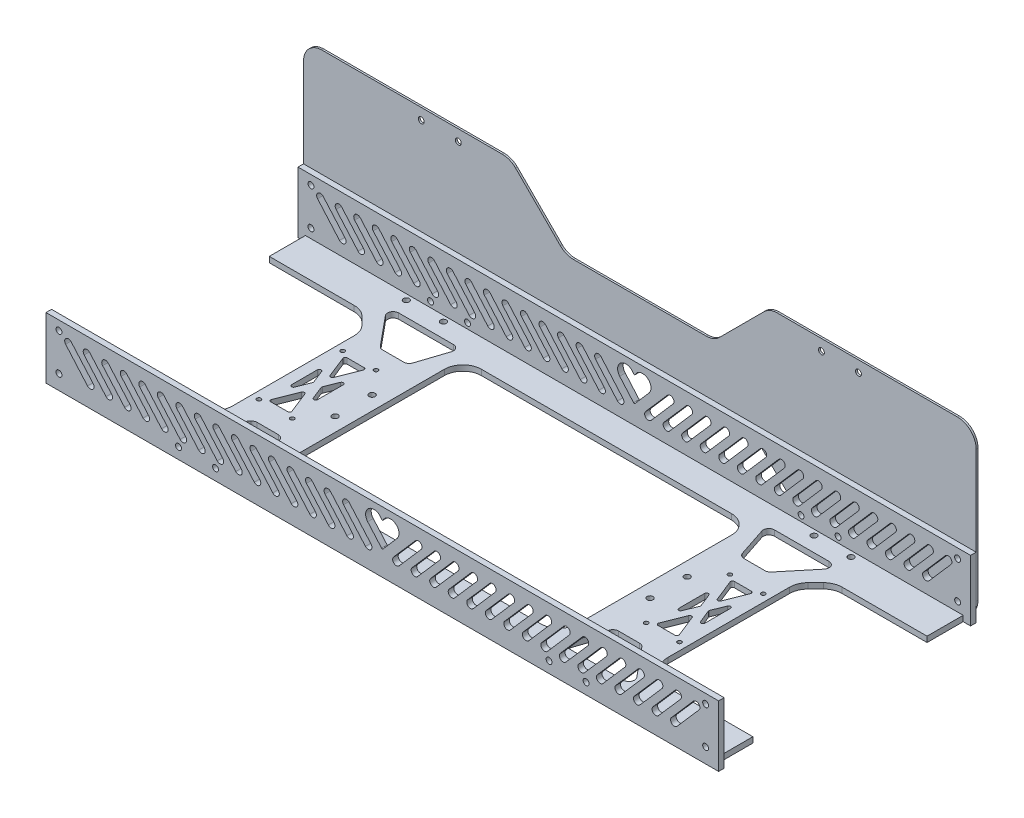
SolidWorks part; units mm, degrees
material "哈碳纤"
ref_plane "前视基准面" through (0, 0, 0) normal (0, 0, 1) x (1, 0, 0)
ref_plane "上视基准面" through (0, 0, 0) normal (0, 1, 0) x (1, 0, 0)
ref_plane "右视基准面" through (0, 0, 0) normal (1, 0, 0) x (0, 0, -1)
other "Configuration Table"
sketch "草图1" plane through (0, 0, 0) normal (0, 1, 0) x (1, 0, 0)
  line L0 (0, 66.5) -> (0, -66.5) construction
  line L1 (-177.5, -66.5) -> (177.5, -66.5)
  line L2 (-177.5, -66.5) -> (-177.5, 66.5)
  line L3 (-177.5, 66.5) -> (177.5, 66.5)
  line L4 (177.5, -66.5) -> (177.5, 66.5)
  line L5 (-177.5, -66.5) -> (177.5, 66.5) construction
  line L6 (-177.5, 66.5) -> (177.5, -66.5) construction
  line L7 (-1000, 0) -> (49000, 0) construction
  circle A4 centre (-120, -63.5) radius 1.6
  circle A5 centre (120, -63.5) radius 1.6
  circle A6 centre (-100, -63.5) radius 1.6
  circle A7 centre (100, -63.5) radius 1.6
  circle A8 centre (100, 63.5) radius 1.6
  circle A9 centre (-100, 63.5) radius 1.6
  circle A10 centre (120, 63.5) radius 1.6
  circle A11 centre (-120, 63.5) radius 1.6
  point P0 (0, 0)
  dimension "D3" = 3
  dimension "D4" = 3.2
  dimension "D1" = 133
  dimension "D2" = 355
  dimension "D5" = 20
  dimension "D6" = 200
extrude "凸台-拉伸1" add sketch "草图1" along normal blind 3
sketch "草图2" plane through (0, 0, 66.5) normal (0, 0, 1) x (1, 0, 0)
  line L1 (-181.5, 0) -> (181.5, 0)
  line L2 (-181.5, 0) -> (-181.5, 33)
  line L3 (-181.5, 33) -> (181.5, 33)
  line L4 (181.5, 0) -> (181.5, 33)
  line L5 (0, 0) -> (0, 33) construction
  line L7 (-100, 3) -> (-100, 0) construction
  line L8 (-177.5, 0) -> (177.5, 0) construction
  circle A0 centre (-174.5, 28) radius 1.6
  circle A1 centre (174.5, 28) radius 1.6
  circle A2 centre (-174.5, 8) radius 1.6
  circle A3 centre (174.5, 8) radius 1.6
  circle A4 centre (-110, 6) radius 1.6
  circle A5 centre (110, 6) radius 1.6
  circle A6 centre (-90, 6) radius 1.6
  circle A7 centre (90, 6) radius 1.6
  dimension "D2" = 7
  dimension "D3" = 3.2
  dimension "D6" = 6
  dimension "D7" = 3.2
  dimension "D1" = 33
  dimension "D4" = 20
  dimension "D5" = 8
  dimension "D8" = 20
  dimension "D9" = 10
  dimension "D10" = 363
extrude "凸台-拉伸2" add sketch "草图2" along normal blind 3 separate body
mirror "镜向1" about plane through (0, 0, 0) normal (0, 0, 1) of bodies 107
sketch "草图3" plane through (0, 3, 0) normal (0, 1, 0) x (1, 0, 0)
  line L0 (0, -1000) -> (0, 49000) construction
  line L1 (-177.5, 47) -> (-127.5, 47)
  line L2 (-177.5, 66.5) -> (-177.5, -66.5) construction
  line L3 (177.5, 47) -> (127.5, 47)
  line L4 (-127.5, 47) -> (-117.5, 37)
  line L5 (127.5, 47) -> (117.5, 37)
  line L6 (-117.5, 37) -> (-117.5, -37)
  line L7 (117.5, 37) -> (117.5, -37)
  line L8 (-117.5, -37) -> (-127.5, -47)
  line L9 (117.5, -37) -> (127.5, -47)
  line L10 (-127.5, -47) -> (-177.5, -47)
  line L11 (127.5, -47) -> (177.5, -47)
  line L12 (-177.5, -47) -> (-177.5, 47)
  line L13 (177.5, -47) -> (177.5, 47)
  line L14 (-177.5, -66.5) -> (177.5, -66.5) construction
  line L15 (-67.5, -51.5) -> (67.5, -51.5)
  line L16 (-77.5, -41.5) -> (-77.5, 41.5)
  line L17 (-67.5, 51.5) -> (67.5, 51.5)
  line L18 (77.5, -41.5) -> (77.5, 41.5)
  line L19 (-77.5, -51.5) -> (77.5, 51.5) construction
  line L20 (-77.5, 51.5) -> (77.5, -51.5) construction
  line L21 (181.5, -66.5) -> (-181.5, -66.5) construction
  line L22 (-85, 10) -> (-85, -10) construction
  line L23 (85, 10) -> (85, -10) construction
  line L24 (95.5, -22.6) -> (95.5, 22.6) construction
  line L25 (-113.5, -22.6) -> (-95.5, -22.6) construction
  line L26 (-113.5, -22.6) -> (-113.5, 22.6) construction
  line L27 (-113.5, 22.6) -> (-95.5, 22.6) construction
  line L28 (-95.5, -22.6) -> (-95.5, 22.6) construction
  line L29 (113.5, 22.6) -> (95.5, 22.6) construction
  line L30 (113.5, -22.6) -> (113.5, 22.6) construction
  line L31 (113.5, -22.6) -> (95.5, -22.6) construction
  arc A0 (-67.5, -51.5) -> (-77.5, -41.5) centre (-67.5, -41.5) cw
  arc A1 (-77.5, 41.5) -> (-67.5, 51.5) centre (-67.5, 41.5) cw
  arc A2 (67.5, 51.5) -> (77.5, 41.5) centre (67.5, 41.5) cw
  arc A3 (67.5, -51.5) -> (77.5, -41.5) centre (67.5, -41.5) ccw
  circle A4 centre (-85, 10) radius 1.6
  circle A5 centre (-85, -10) radius 1.6
  circle A6 centre (85, -10) radius 1.6
  circle A7 centre (85, 10) radius 1.6
  circle A8 centre (-113.5, 22.6) radius 1.1
  circle A9 centre (-95.5, 22.6) radius 1.1
  circle A11 centre (-113.5, -22.6) radius 1.1
  circle A12 centre (-95.5, -22.6) radius 1.1
  circle A13 centre (95.5, -22.6) radius 1.1
  circle A14 centre (113.5, -22.6) radius 1.1
  circle A15 centre (95.5, 22.6) radius 1.1
  circle A16 centre (113.5, 22.6) radius 1.1
  point P17 (-177.5, 0)
  point P18 (0, 0)
  point P43 (-85, 0)
  point P52 (-95.5, 0)
  dimension "D6" = 10
  dimension "D7" = 3.2
  dimension "D13" = 2.2
  dimension "D1" = 19.5
  dimension "D2" = 60
  dimension "D3" = 50
  dimension "D4" = 40
  dimension "D5" = 15
  dimension "D8" = 20
  dimension "D9" = 170
  dimension "D10" = 45.2
  dimension "D11" = 18
  dimension "D12" = 4
extrude "切除-拉伸1" cut sketch "草图3" against normal blind 10
fillet "圆角1" radius 10 8 edges at (127.5, 1.5, 47) (117.5, 1.5, 37) (117.5, 1.5, -37) (-127.5, 1.5, 47) (-117.5, 1.5, 37) (-117.5, 1.5, -37) (-127.5, 1.5, -47) (127.5, 1.5, -47)
sketch "草图4" plane through (0, 0, 69.5) normal (0, 0, 1) x (1, 0, 0)
  line L0 (-169.4178, 24.7808) -> (-157.5822, 11.2192) construction
  line L1 (-167.911, 26.0959) -> (-156.0753, 12.5342)
  line L2 (-170.9247, 23.4658) -> (-159.089, 9.9041)
  line L3 (181.5, 33) -> (-181.5, 33) construction
  line L4 (-181.5, 33) -> (-181.5, 0) construction
  line L5 (-181.5, 0) -> (181.5, 0) construction
  line L6 (-159.4178, 24.7808) -> (-147.5822, 11.2192) construction
  line L7 (-157.911, 26.0959) -> (-146.0753, 12.5342)
  line L8 (-160.9247, 23.4658) -> (-149.089, 9.9041)
  line L9 (-149.4178, 24.7808) -> (-137.5822, 11.2192) construction
  line L10 (-147.911, 26.0959) -> (-136.0753, 12.5342)
  line L11 (-150.9247, 23.4658) -> (-139.089, 9.9041)
  line L12 (-139.4178, 24.7808) -> (-127.5822, 11.2192) construction
  line L13 (-137.911, 26.0959) -> (-126.0753, 12.5342)
  line L14 (-140.9247, 23.4658) -> (-129.089, 9.9041)
  line L15 (-129.4178, 24.7808) -> (-117.5822, 11.2192) construction
  line L16 (-127.911, 26.0959) -> (-116.0753, 12.5342)
  line L17 (-130.9247, 23.4658) -> (-119.089, 9.9041)
  line L18 (-119.4178, 24.7808) -> (-107.5822, 11.2192) construction
  line L19 (-117.911, 26.0959) -> (-106.0753, 12.5342)
  line L20 (-120.9247, 23.4658) -> (-109.089, 9.9041)
  line L21 (-109.4178, 24.7808) -> (-97.5822, 11.2192) construction
  line L22 (-107.911, 26.0959) -> (-96.0753, 12.5342)
  line L23 (-110.9247, 23.4658) -> (-99.089, 9.9041)
  line L24 (-99.4178, 24.7808) -> (-87.5822, 11.2192) construction
  line L25 (-97.911, 26.0959) -> (-86.0753, 12.5342)
  line L26 (-100.9247, 23.4658) -> (-89.089, 9.9041)
  line L27 (-89.4178, 24.7808) -> (-77.5822, 11.2192) construction
  line L28 (-87.911, 26.0959) -> (-76.0753, 12.5342)
  line L29 (-90.9247, 23.4658) -> (-79.089, 9.9041)
  line L30 (-79.4178, 24.7808) -> (-67.5822, 11.2192) construction
  line L31 (-77.911, 26.0959) -> (-66.0753, 12.5342)
  line L32 (-80.9247, 23.4658) -> (-69.089, 9.9041)
  line L33 (-69.4178, 24.7808) -> (-57.5822, 11.2192) construction
  line L34 (-67.911, 26.0959) -> (-56.0753, 12.5342)
  line L35 (-70.9247, 23.4658) -> (-59.089, 9.9041)
  line L36 (-59.4178, 24.7808) -> (-47.5822, 11.2192) construction
  line L37 (-57.911, 26.0959) -> (-46.0753, 12.5342)
  line L38 (-60.9247, 23.4658) -> (-49.089, 9.9041)
  line L39 (-49.4178, 24.7808) -> (-37.5822, 11.2192) construction
  line L40 (-47.911, 26.0959) -> (-36.0753, 12.5342)
  line L41 (-50.9247, 23.4658) -> (-39.089, 9.9041)
  line L42 (-39.4178, 24.7808) -> (-27.5822, 11.2192) construction
  line L43 (-37.911, 26.0959) -> (-26.0753, 12.5342)
  line L44 (-40.9247, 23.4658) -> (-29.089, 9.9041)
  line L45 (-29.4178, 24.7808) -> (-17.5822, 11.2192) construction
  line L46 (-27.911, 26.0959) -> (-16.0753, 12.5342)
  line L47 (-30.9247, 23.4658) -> (-19.089, 9.9041)
  line L48 (-19.4178, 24.7808) -> (-7.5822, 11.2192) construction
  line L49 (-17.911, 26.0959) -> (-6.0753, 12.5342)
  line L50 (-20.9247, 23.4658) -> (-9.089, 9.9041)
  line L51 (-169.4178, 24.7808) -> (-159.4178, 24.7808) construction
  line L52 (0, 33) -> (0, 0) construction
  line L53 (169.4178, 24.7808) -> (157.5822, 11.2192) construction
  line L54 (167.911, 26.0959) -> (156.0753, 12.5342)
  line L55 (170.9247, 23.4658) -> (159.089, 9.9041)
  line L56 (159.4178, 24.7808) -> (147.5822, 11.2192) construction
  line L57 (157.911, 26.0959) -> (146.0753, 12.5342)
  line L58 (160.9247, 23.4658) -> (149.089, 9.9041)
  line L59 (149.4178, 24.7808) -> (137.5822, 11.2192) construction
  line L60 (147.911, 26.0959) -> (136.0753, 12.5342)
  line L61 (150.9247, 23.4658) -> (139.089, 9.9041)
  line L62 (139.4178, 24.7808) -> (127.5822, 11.2192) construction
  line L63 (137.911, 26.0959) -> (126.0753, 12.5342)
  line L64 (140.9247, 23.4658) -> (129.089, 9.9041)
  line L65 (129.4178, 24.7808) -> (117.5822, 11.2192) construction
  line L66 (127.911, 26.0959) -> (116.0753, 12.5342)
  line L67 (130.9247, 23.4658) -> (119.089, 9.9041)
  line L68 (119.4178, 24.7808) -> (107.5822, 11.2192) construction
  line L69 (117.911, 26.0959) -> (106.0753, 12.5342)
  line L70 (120.9247, 23.4658) -> (109.089, 9.9041)
  line L71 (109.4178, 24.7808) -> (97.5822, 11.2192) construction
  line L72 (107.911, 26.0959) -> (96.0753, 12.5342)
  line L73 (110.9247, 23.4658) -> (99.089, 9.9041)
  line L74 (99.4178, 24.7808) -> (87.5822, 11.2192) construction
  line L75 (97.911, 26.0959) -> (86.0753, 12.5342)
  line L76 (100.9247, 23.4658) -> (89.089, 9.9041)
  line L77 (89.4178, 24.7808) -> (77.5822, 11.2192) construction
  line L78 (87.911, 26.0959) -> (76.0753, 12.5342)
  line L79 (90.9247, 23.4658) -> (79.089, 9.9041)
  line L80 (79.4178, 24.7808) -> (67.5822, 11.2192) construction
  line L81 (77.911, 26.0959) -> (66.0753, 12.5342)
  line L82 (80.9247, 23.4658) -> (69.089, 9.9041)
  line L83 (69.4178, 24.7808) -> (57.5822, 11.2192) construction
  line L84 (67.911, 26.0959) -> (56.0753, 12.5342)
  line L85 (70.9247, 23.4658) -> (59.089, 9.9041)
  line L86 (59.4178, 24.7808) -> (47.5822, 11.2192) construction
  line L87 (57.911, 26.0959) -> (46.0753, 12.5342)
  line L88 (60.9247, 23.4658) -> (49.089, 9.9041)
  line L89 (49.4178, 24.7808) -> (37.5822, 11.2192) construction
  line L90 (47.911, 26.0959) -> (36.0753, 12.5342)
  line L91 (50.9247, 23.4658) -> (39.089, 9.9041)
  line L92 (39.4178, 24.7808) -> (27.5822, 11.2192) construction
  line L93 (37.911, 26.0959) -> (26.0753, 12.5342)
  line L94 (40.9247, 23.4658) -> (29.089, 9.9041)
  line L95 (29.4178, 24.7808) -> (17.5822, 11.2192) construction
  line L96 (27.911, 26.0959) -> (16.0753, 12.5342)
  line L97 (30.9247, 23.4658) -> (19.089, 9.9041)
  line L98 (19.4178, 24.7808) -> (7.5822, 11.2192) construction
  line L99 (17.911, 26.0959) -> (6.0753, 12.5342)
  line L100 (20.9247, 23.4658) -> (9.089, 9.9041)
  line L101 (169.4178, 24.7808) -> (159.4178, 24.7808) construction
  line L102 (-0.3767, 13.4316) -> (-7.8904, 22.0411)
  line L103 (0.3767, 13.4316) -> (7.8904, 22.0411)
  arc A0 (-167.911, 26.0959) -> (-170.9247, 23.4658) centre (-169.4178, 24.7808) ccw
  arc A1 (-159.089, 9.9041) -> (-156.0753, 12.5342) centre (-157.5822, 11.2192) ccw
  arc A2 (-157.911, 26.0959) -> (-160.9247, 23.4658) centre (-159.4178, 24.7808) ccw
  arc A3 (-149.089, 9.9041) -> (-146.0753, 12.5342) centre (-147.5822, 11.2192) ccw
  arc A4 (-147.911, 26.0959) -> (-150.9247, 23.4658) centre (-149.4178, 24.7808) ccw
  arc A5 (-139.089, 9.9041) -> (-136.0753, 12.5342) centre (-137.5822, 11.2192) ccw
  arc A6 (-137.911, 26.0959) -> (-140.9247, 23.4658) centre (-139.4178, 24.7808) ccw
  arc A7 (-129.089, 9.9041) -> (-126.0753, 12.5342) centre (-127.5822, 11.2192) ccw
  arc A8 (-127.911, 26.0959) -> (-130.9247, 23.4658) centre (-129.4178, 24.7808) ccw
  arc A9 (-119.089, 9.9041) -> (-116.0753, 12.5342) centre (-117.5822, 11.2192) ccw
  arc A10 (-117.911, 26.0959) -> (-120.9247, 23.4658) centre (-119.4178, 24.7808) ccw
  arc A11 (-109.089, 9.9041) -> (-106.0753, 12.5342) centre (-107.5822, 11.2192) ccw
  arc A12 (-107.911, 26.0959) -> (-110.9247, 23.4658) centre (-109.4178, 24.7808) ccw
  arc A13 (-99.089, 9.9041) -> (-96.0753, 12.5342) centre (-97.5822, 11.2192) ccw
  arc A14 (-97.911, 26.0959) -> (-100.9247, 23.4658) centre (-99.4178, 24.7808) ccw
  arc A15 (-89.089, 9.9041) -> (-86.0753, 12.5342) centre (-87.5822, 11.2192) ccw
  arc A16 (-87.911, 26.0959) -> (-90.9247, 23.4658) centre (-89.4178, 24.7808) ccw
  arc A17 (-79.089, 9.9041) -> (-76.0753, 12.5342) centre (-77.5822, 11.2192) ccw
  arc A18 (-77.911, 26.0959) -> (-80.9247, 23.4658) centre (-79.4178, 24.7808) ccw
  arc A19 (-69.089, 9.9041) -> (-66.0753, 12.5342) centre (-67.5822, 11.2192) ccw
  arc A20 (-67.911, 26.0959) -> (-70.9247, 23.4658) centre (-69.4178, 24.7808) ccw
  arc A21 (-59.089, 9.9041) -> (-56.0753, 12.5342) centre (-57.5822, 11.2192) ccw
  arc A22 (-57.911, 26.0959) -> (-60.9247, 23.4658) centre (-59.4178, 24.7808) ccw
  arc A23 (-49.089, 9.9041) -> (-46.0753, 12.5342) centre (-47.5822, 11.2192) ccw
  arc A24 (-47.911, 26.0959) -> (-50.9247, 23.4658) centre (-49.4178, 24.7808) ccw
  arc A25 (-39.089, 9.9041) -> (-36.0753, 12.5342) centre (-37.5822, 11.2192) ccw
  arc A26 (-37.911, 26.0959) -> (-40.9247, 23.4658) centre (-39.4178, 24.7808) ccw
  arc A27 (-29.089, 9.9041) -> (-26.0753, 12.5342) centre (-27.5822, 11.2192) ccw
  arc A28 (-27.911, 26.0959) -> (-30.9247, 23.4658) centre (-29.4178, 24.7808) ccw
  arc A29 (-19.089, 9.9041) -> (-16.0753, 12.5342) centre (-17.5822, 11.2192) ccw
  arc A30 (-17.911, 26.0959) -> (-20.9247, 23.4658) centre (-19.4178, 24.7808) ccw
  arc A31 (-9.089, 9.9041) -> (-6.0753, 12.5342) centre (-7.5822, 11.2192) ccw
  arc A32 (167.911, 26.0959) -> (170.9247, 23.4658) centre (169.4178, 24.7808) cw
  arc A33 (159.089, 9.9041) -> (156.0753, 12.5342) centre (157.5822, 11.2192) cw
  arc A34 (157.911, 26.0959) -> (160.9247, 23.4658) centre (159.4178, 24.7808) cw
  arc A35 (149.089, 9.9041) -> (146.0753, 12.5342) centre (147.5822, 11.2192) cw
  arc A36 (147.911, 26.0959) -> (150.9247, 23.4658) centre (149.4178, 24.7808) cw
  arc A37 (139.089, 9.9041) -> (136.0753, 12.5342) centre (137.5822, 11.2192) cw
  arc A38 (137.911, 26.0959) -> (140.9247, 23.4658) centre (139.4178, 24.7808) cw
  arc A39 (129.089, 9.9041) -> (126.0753, 12.5342) centre (127.5822, 11.2192) cw
  arc A40 (127.911, 26.0959) -> (130.9247, 23.4658) centre (129.4178, 24.7808) cw
  arc A41 (119.089, 9.9041) -> (116.0753, 12.5342) centre (117.5822, 11.2192) cw
  arc A42 (117.911, 26.0959) -> (120.9247, 23.4658) centre (119.4178, 24.7808) cw
  arc A43 (109.089, 9.9041) -> (106.0753, 12.5342) centre (107.5822, 11.2192) cw
  arc A44 (107.911, 26.0959) -> (110.9247, 23.4658) centre (109.4178, 24.7808) cw
  arc A45 (99.089, 9.9041) -> (96.0753, 12.5342) centre (97.5822, 11.2192) cw
  arc A46 (97.911, 26.0959) -> (100.9247, 23.4658) centre (99.4178, 24.7808) cw
  arc A47 (89.089, 9.9041) -> (86.0753, 12.5342) centre (87.5822, 11.2192) cw
  arc A48 (87.911, 26.0959) -> (90.9247, 23.4658) centre (89.4178, 24.7808) cw
  arc A49 (79.089, 9.9041) -> (76.0753, 12.5342) centre (77.5822, 11.2192) cw
  arc A50 (77.911, 26.0959) -> (80.9247, 23.4658) centre (79.4178, 24.7808) cw
  arc A51 (69.089, 9.9041) -> (66.0753, 12.5342) centre (67.5822, 11.2192) cw
  arc A52 (67.911, 26.0959) -> (70.9247, 23.4658) centre (69.4178, 24.7808) cw
  arc A53 (59.089, 9.9041) -> (56.0753, 12.5342) centre (57.5822, 11.2192) cw
  arc A54 (57.911, 26.0959) -> (60.9247, 23.4658) centre (59.4178, 24.7808) cw
  arc A55 (49.089, 9.9041) -> (46.0753, 12.5342) centre (47.5822, 11.2192) cw
  arc A56 (47.911, 26.0959) -> (50.9247, 23.4658) centre (49.4178, 24.7808) cw
  arc A57 (39.089, 9.9041) -> (36.0753, 12.5342) centre (37.5822, 11.2192) cw
  arc A58 (37.911, 26.0959) -> (40.9247, 23.4658) centre (39.4178, 24.7808) cw
  arc A59 (29.089, 9.9041) -> (26.0753, 12.5342) centre (27.5822, 11.2192) cw
  arc A60 (27.911, 26.0959) -> (30.9247, 23.4658) centre (29.4178, 24.7808) cw
  arc A61 (19.089, 9.9041) -> (16.0753, 12.5342) centre (17.5822, 11.2192) cw
  arc A62 (17.911, 26.0959) -> (20.9247, 23.4658) centre (19.4178, 24.7808) cw
  arc A63 (9.089, 9.9041) -> (6.0753, 12.5342) centre (7.5822, 11.2192) cw
  arc A64 (-0.45, 26.9615) -> (-7.8904, 22.0411) centre (-4.5, 25) ccw
  arc A65 (0.45, 26.9615) -> (7.8904, 22.0411) centre (4.5, 25) cw
  arc A66 (-0.3767, 13.4316) -> (0.3767, 13.4316) centre (0, 13.7604) ccw
  arc A67 (0.45, 26.9615) -> (-0.45, 26.9615) centre (0, 27.1794) cw
  point P2 (-163.5, 18)
  point P16 (-153.5, 18)
  point P23 (-143.5, 18)
  point P30 (-133.5, 18)
  point P37 (-123.5, 18)
  point P44 (-113.5, 18)
  point P51 (-103.5, 18)
  point P58 (-93.5, 18)
  point P65 (-83.5, 18)
  point P72 (-73.5, 18)
  point P79 (-63.5, 18)
  point P86 (-53.5, 18)
  point P93 (-43.5, 18)
  point P100 (-33.5, 18)
  point P107 (-23.5, 18)
  point P114 (-13.5, 18)
  point P125 (163.5, 18)
  point P132 (153.5, 18)
  point P139 (143.5, 18)
  point P146 (133.5, 18)
  point P153 (123.5, 18)
  point P160 (113.5, 18)
  point P167 (103.5, 18)
  point P174 (93.5, 18)
  point P181 (83.5, 18)
  point P188 (73.5, 18)
  point P195 (63.5, 18)
  point P202 (53.5, 18)
  point P209 (43.5, 18)
  point P216 (33.5, 18)
  point P223 (23.5, 18)
  point P230 (13.5, 18)
  point P243 (0, 13)
  point P248 (0, 25)
extrude "切除-拉伸2" cut sketch "草图4" against normal through all
sketch "草图6" plane through (0, 3, 0) normal (0, 1, 0) x (1, 0, 0)
  line L0 (-109.0762, -20.6) -> (-99.9238, -20.6)
  line L1 (-113.5, -22.6) -> (-95.5, -22.6) construction
  line L2 (-113.5, -22.6) -> (-113.5, 22.6) construction
  line L3 (-113.5, 22.6) -> (-95.5, 22.6) construction
  line L4 (-95.5, -22.6) -> (-95.5, 22.6) construction
  line L5 (-113.5, -22.6) -> (-95.5, 22.6) construction
  line L6 (-113.5, 22.6) -> (-95.5, -22.6) construction
  line L7 (-111.5, -6.958) -> (-111.5, 6.958)
  line L9 (-110.0052, -19.23) -> (-105.429, -7.7387)
  line L10 (-103.571, 7.7387) -> (-98.9948, 19.23)
  line L11 (-109.571, 7.3279) -> (-106.8001, 0.37)
  line L12 (-102.1999, 0.37) -> (-99.429, 7.3279)
  line L13 (-111.6419, 23.3399) -> (-93.6419, -21.8601) construction
  line L14 (-115.3581, -21.8601) -> (-97.3581, 23.3399) construction
  line L15 (-102.1999, -0.37) -> (-99.429, -7.3279)
  line L16 (-109.571, -7.3279) -> (-106.8001, -0.37)
  line L17 (-110.0052, 19.23) -> (-105.429, 7.7387)
  line L18 (-111.5, -22.6) -> (-111.5, 22.6) construction
  line L19 (-115.3581, 21.8601) -> (-97.3581, -23.3399) construction
  line L20 (-109.0762, 20.6) -> (-99.9238, 20.6)
  line L22 (-97.5, -6.958) -> (-97.5, 6.958)
  line L23 (-103.571, -7.7387) -> (-98.9948, -19.23)
  line L24 (-117.5, 32.8579) -> (-77.5, 32.8579) construction
  line L25 (-118.4432, 50.5893) -> (-105.5208, 34.9472)
  line L26 (-103.208, 33.8579) -> (-91.792, 33.8579)
  line L27 (-88.9423, 35.9202) -> (-83.7956, 51.5624)
  line L28 (-86.6453, 55.5) -> (-116.1303, 55.5)
  line L29 (-177.5, 66.5) -> (-177.5, 47) construction
  line L30 (-77.5, 41.5) -> (-77.5, -41.5) construction
  line L31 (-103.208, -33.8579) -> (-91.792, -33.8579)
  line L32 (-95.5, 0) -> (95.5, 0) construction
  line L33 (-86.6453, -55.5) -> (-116.1303, -55.5)
  line L34 (-88.9423, -35.9202) -> (-83.7956, -51.5624)
  line L35 (-118.4432, -50.5893) -> (-105.5208, -34.9472)
  line L36 (0, 0) -> (0, -51.5) construction
  line L37 (-67.5, -51.5) -> (67.5, -51.5) construction
  line L38 (117.5, 32.8579) -> (77.5, 32.8579) construction
  line L39 (113.5, 22.6) -> (97.429, -17.756) construction
  line L40 (111.571, -17.756) -> (96.0456, 21.23) construction
  line L41 (95.5, -17.386) -> (95.5, 22.6) construction
  line L42 (112.5, 22.6) -> (96.9746, 22.6) construction
  line L43 (113.5, -17.386) -> (113.5, 21.6) construction
  line L44 (113.5, -22.6) -> (95.5, -22.6) construction
  line L45 (118.4432, -50.5893) -> (105.5208, -34.9472)
  line L46 (88.9423, -35.9202) -> (83.7956, -51.5624)
  line L47 (86.6453, -55.5) -> (116.1303, -55.5)
  line L48 (103.208, -33.8579) -> (91.792, -33.8579)
  line L49 (86.6453, 55.5) -> (116.1303, 55.5)
  line L50 (88.9423, 35.9202) -> (83.7956, 51.5624)
  line L51 (103.208, 33.8579) -> (91.792, 33.8579)
  line L52 (118.4432, 50.5893) -> (105.5208, 34.9472)
  line L53 (103.571, -7.7387) -> (98.9948, -19.23)
  line L54 (97.5, -6.958) -> (97.5, 6.958)
  line L55 (109.0762, 20.6) -> (99.9238, 20.6)
  line L56 (110.0052, 19.23) -> (105.429, 7.7387)
  line L57 (109.571, -7.3279) -> (106.8001, -0.37)
  line L58 (102.1999, -0.37) -> (99.429, -7.3279)
  line L59 (102.1999, 0.37) -> (99.429, 7.3279)
  line L60 (109.571, 7.3279) -> (106.8001, 0.37)
  line L61 (103.571, 7.7387) -> (98.9948, 19.23)
  line L62 (110.0052, -19.23) -> (105.429, -7.7387)
  line L64 (111.5, -6.958) -> (111.5, 6.958)
  line L65 (109.0762, -20.6) -> (99.9238, -20.6)
  arc A0 (83.7956, -51.5624) -> (86.6453, -55.5) centre (86.6453, -52.5) ccw
  arc A1 (88.9423, -35.9202) -> (91.792, -33.8579) centre (91.792, -36.8579) cw
  arc A2 (105.5208, -34.9472) -> (103.208, -33.8579) centre (103.208, -36.8579) ccw
  arc A3 (118.4432, -50.5893) -> (116.1303, -55.5) centre (116.1303, -52.5) cw
  arc A4 (-116.1303, -55.5) -> (-118.4432, -50.5893) centre (-116.1303, -52.5) cw
  arc A5 (-86.6453, -55.5) -> (-83.7956, -51.5624) centre (-86.6453, -52.5) ccw
  arc A6 (-91.792, -33.8579) -> (-88.9423, -35.9202) centre (-91.792, -36.8579) cw
  arc A7 (-103.208, -33.8579) -> (-105.5208, -34.9472) centre (-103.208, -36.8579) ccw
  arc A8 (103.208, 33.8579) -> (105.5208, 34.9472) centre (103.208, 36.8579) ccw
  arc A9 (88.9423, 35.9202) -> (91.792, 33.8579) centre (91.792, 36.8579) ccw
  arc A10 (116.1303, 55.5) -> (118.4432, 50.5893) centre (116.1303, 52.5) cw
  arc A11 (86.6453, 55.5) -> (83.7956, 51.5624) centre (86.6453, 52.5) ccw
  arc A12 (-83.7956, 51.5624) -> (-86.6453, 55.5) centre (-86.6453, 52.5) ccw
  arc A13 (-105.5208, 34.9472) -> (-103.208, 33.8579) centre (-103.208, 36.8579) ccw
  arc A14 (-118.4432, 50.5893) -> (-116.1303, 55.5) centre (-116.1303, 52.5) cw
  arc A15 (-91.792, 33.8579) -> (-88.9423, 35.9202) centre (-91.792, 36.8579) ccw
  arc A16 (110.0052, -19.23) -> (109.0762, -20.6) centre (109.0762, -19.6) cw
  arc A17 (109.571, 7.3279) -> (111.5, 6.958) centre (110.5, 6.958) cw
  arc A18 (102.1999, -0.37) -> (102.1999, 0.37) centre (101.2709, 0) ccw
  arc A19 (106.8001, -0.37) -> (106.8001, 0.37) centre (107.7291, 0) cw
  arc A20 (109.571, -7.3279) -> (111.5, -6.958) centre (110.5, -6.958) ccw
  arc A21 (105.429, 7.7387) -> (103.571, 7.7387) centre (104.5, 8.1087) cw
  arc A22 (99.9238, 20.6) -> (98.9948, 19.23) centre (99.9238, 19.6) ccw
  arc A23 (109.0762, 20.6) -> (110.0052, 19.23) centre (109.0762, 19.6) cw
  arc A24 (97.5, 6.958) -> (99.429, 7.3279) centre (98.5, 6.958) cw
  arc A25 (97.5, -6.958) -> (99.429, -7.3279) centre (98.5, -6.958) ccw
  arc A26 (98.9948, -19.23) -> (99.9238, -20.6) centre (99.9238, -19.6) ccw
  arc A27 (103.571, -7.7387) -> (105.429, -7.7387) centre (104.5, -8.1087) cw
  arc A28 (96.9746, 22.6) -> (96.0456, 21.23) centre (96.9746, 21.6) ccw construction
  arc A29 (113.5, 21.6) -> (112.5, 22.6) centre (112.5, 21.6) ccw construction
  arc A30 (97.429, -17.756) -> (95.5, -17.386) centre (96.5, -17.386) cw construction
  arc A31 (113.5, -17.386) -> (111.571, -17.756) centre (112.5, -17.386) cw construction
  arc A32 (-102.1999, 0.37) -> (-102.1999, -0.37) centre (-101.2709, 0) ccw
  arc A33 (-110.0052, -19.23) -> (-109.0762, -20.6) centre (-109.0762, -19.6) ccw
  arc A34 (-103.571, 7.7387) -> (-105.429, 7.7387) centre (-104.5, 8.1087) cw
  arc A35 (-99.429, -7.3279) -> (-97.5, -6.958) centre (-98.5, -6.958) ccw
  arc A36 (-98.9948, -19.23) -> (-99.9238, -20.6) centre (-99.9238, -19.6) cw
  arc A37 (-105.429, -7.7387) -> (-103.571, -7.7387) centre (-104.5, -8.1087) cw
  arc A38 (-111.5, -6.958) -> (-109.571, -7.3279) centre (-110.5, -6.958) ccw
  arc A39 (-106.8001, -0.37) -> (-106.8001, 0.37) centre (-107.7291, 0) ccw
  arc A40 (-110.0052, 19.23) -> (-109.0762, 20.6) centre (-109.0762, 19.6) cw
  arc A41 (-98.9948, 19.23) -> (-99.9238, 20.6) centre (-99.9238, 19.6) ccw
  arc A42 (-99.429, 7.3279) -> (-97.5, 6.958) centre (-98.5, 6.958) cw
  arc A43 (-109.571, 7.3279) -> (-111.5, 6.958) centre (-110.5, 6.958) ccw
  point P0 (-104.5, 0)
  point P24 (82.5, -55.5)
  point P40 (-97.5, 32.8579)
  point P41 (-97.5, 33.8579)
  point P83 (104.5, 0)
  point P84 (89.6209, -33.8579)
  point P87 (104.6209, -33.8579)
  point P90 (122.5, -55.5)
  point P93 (-122.5, -55.5)
  point P96 (-82.5, -55.5)
  point P99 (-89.6209, -33.8579)
  point P102 (-104.6209, -33.8579)
  point P105 (104.6209, 33.8579)
  point P108 (89.6209, 33.8579)
  point P111 (122.5, 55.5)
  point P114 (82.5, 55.5)
  point P117 (-82.5, 55.5)
  point P120 (-104.6209, 33.8579)
  point P123 (-122.5, 55.5)
  point P126 (-89.6209, 33.8579)
  point P129 (110.5508, -20.6)
  point P132 (111.5, 12.172)
  point P135 (102.3472, 0)
  point P138 (106.6528, 0)
  point P141 (111.5, -12.172)
  point P144 (104.5, 5.4058)
  point P147 (98.4492, 20.6)
  point P150 (110.5508, 20.6)
  point P153 (97.5, 12.172)
  point P156 (97.5, -12.172)
  point P159 (98.4492, -20.6)
  point P162 (104.5, -5.4058)
  point P177 (-102.3472, 0)
  point P180 (-110.5508, -20.6)
  point P183 (-104.5, 5.4058)
  point P186 (-97.5, -12.172)
  point P189 (-98.4492, -20.6)
  point P192 (-104.5, -5.4058)
  point P195 (-111.5, -12.172)
  point P198 (-106.6528, 0)
  point P201 (-110.5508, 20.6)
  point P204 (-98.4492, 20.6)
  point P207 (-97.5, 12.172)
  point P210 (-111.5, 12.172)
  dimension "D12" = 3
  dimension "D13" = 1
  dimension "D1" = 2
  dimension "D2" = 2
  dimension "D3" = 4
  dimension "D4" = 4
  dimension "D5" = 4
  dimension "D6" = 8
  dimension "D7" = 15
  dimension "D8" = 1
  dimension "D9" = 40
  dimension "D10" = 55
  dimension "D11" = 4
extrude "切除-拉伸3" cut sketch "草图6" against normal blind 10
sketch "草图7" plane through (0, 0, -69.5) normal (0, 0, 1) x (1, 0, 0)
  line L0 (0, -1000) -> (0, 49000) construction
  line L1 (-181.5, 0) -> (-181.5, 91.15)
  line L2 (-181.5, 91.15) -> (-70, 91.15)
  line L3 (-70, 91.15) -> (-40, 61.15)
  line L4 (-40, 61.15) -> (40, 61.15)
  line L6 (58.5, 31) -> (-58.5, 31)
  line L7 (-58.5, 31) -> (-89.5, 0)
  line L8 (-181.5, 0) -> (181.5, 0) construction
  line L9 (-89.5, 0) -> (-181.5, 0)
  line L10 (181.5, 33) -> (-181.5, 33) construction
  line L11 (89.5, 0) -> (181.5, 0)
  line L12 (58.5, 31) -> (89.5, 0)
  line L13 (70, 91.15) -> (40, 61.15)
  line L14 (181.5, 91.15) -> (70, 91.15)
  line L15 (181.5, 0) -> (181.5, 91.15)
  circle A0 centre (-174.5, 28) radius 1.6 construction
  circle A1 centre (-174.5, 8) radius 1.6 construction
  circle A2 centre (-110, 6) radius 1.6 construction
  circle A3 centre (-90, 6) radius 1.6 construction
  circle A4 centre (90, 6) radius 1.6 construction
  circle A5 centre (110, 6) radius 1.6 construction
  circle A6 centre (174.5, 8) radius 1.6 construction
  circle A7 centre (174.5, 28) radius 1.6 construction
  circle A8 centre (-174.5, 28) radius 1.6
  circle A9 centre (-174.5, 8) radius 1.6
  circle A10 centre (-110, 6) radius 1.6
  circle A11 centre (-90, 6) radius 1.6
  circle A12 centre (90, 6) radius 1.6
  circle A13 centre (110, 6) radius 1.6
  circle A14 centre (174.5, 8) radius 1.6
  circle A15 centre (174.5, 28) radius 1.6
  circle A16 centre (118, 85.15) radius 1.6
  circle A17 centre (98, 85.15) radius 1.6
  circle A20 centre (-98, 85.15) radius 1.6
  circle A21 centre (-118, 85.15) radius 1.6
  point P19 (0, 31)
  point P20 (0, 61.15)
  point P50 (0, 0)
  point P51 (0, 0)
  dimension "D8" = 20
  dimension "D10" = 3.2
  dimension "D1" = 91.15
  dimension "D2" = 2
  dimension "D3" = 92
  dimension "D4" = 30
  dimension "D5" = 45
  dimension "D6" = 45
  dimension "D7" = 140
  dimension "D9" = 6
  dimension "D11" = 196
extrude "凸台-拉伸3" add sketch "草图7" against normal blind 1 separate body
fillet "圆角2" radius 10 12 edges at (-89.5, 0, -70) (-58.5, 31, -70) (58.5, 31, -70) (89.5, 0, -70) (181.5, 0, -70) (181.5, 91.15, -70) (40, 61.15, -70) (-40, 61.15, -70) (-70, 91.15, -70) (-181.5, 91.15, -70) (-181.5, 0, -70) (70, 91.15, -70)
equation "\"D5@草图4\"=\"D11@草图4\""
